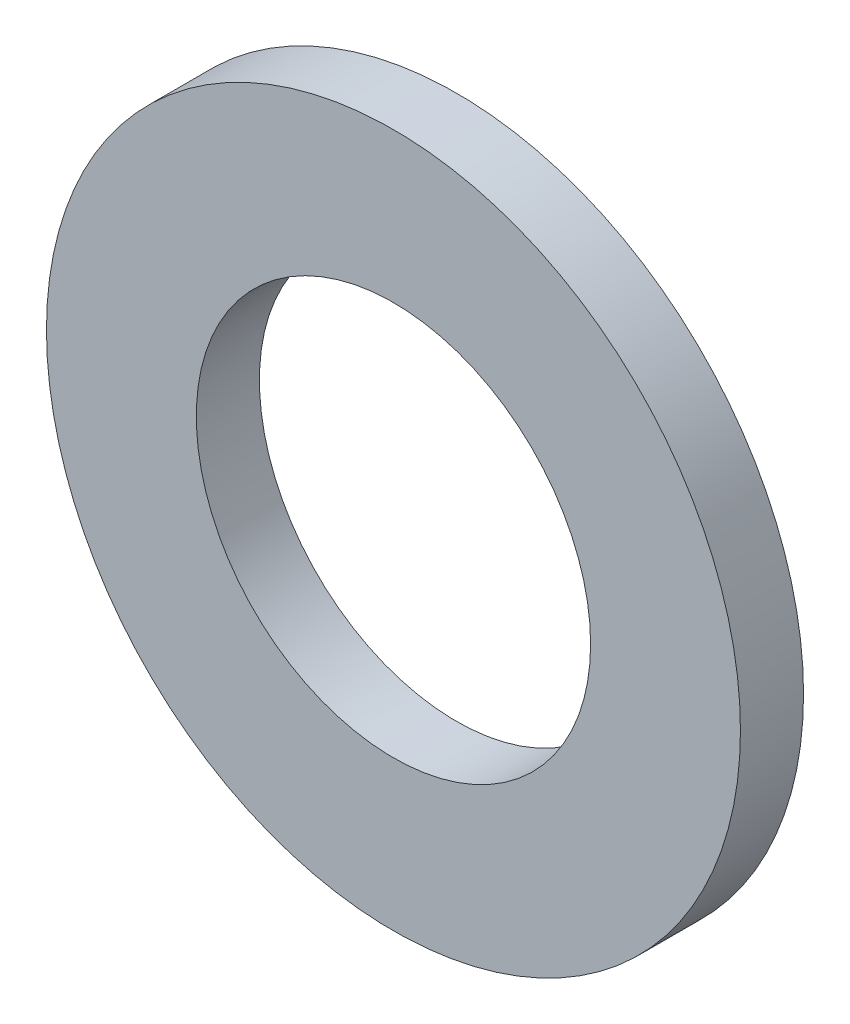
from build123d import *

# Parameters (mm, degrees)
SKETCH_246_R    = 22
SKETCH_246_R_2  = 12.5
EXTRUDE_1_DEPTH = 4


with BuildPart() as part:
    # Sketch 246 → 拉伸1 (new body)
    with BuildSketch(Plane.XY):
        Circle(SKETCH_246_R)
        Circle(SKETCH_246_R_2, mode=Mode.SUBTRACT)
    extrude(amount=EXTRUDE_1_DEPTH)


solid = part.part
